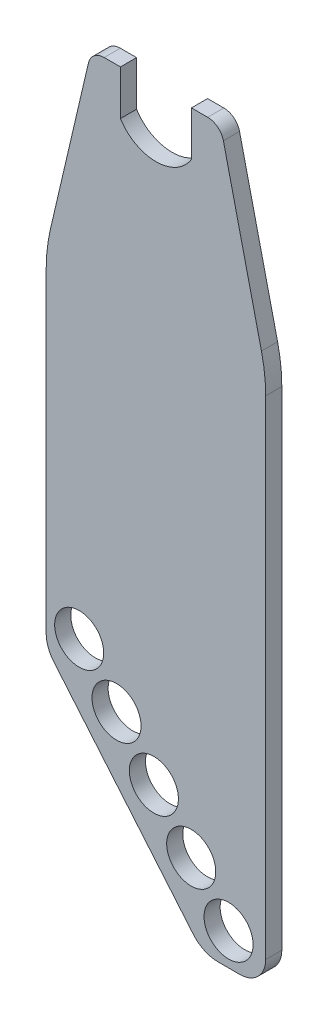
from build123d import *

# Parameters (mm, degrees)
SKETCH1_W           = 68
SKETCH1_H           = 225
BOSS_EXTRUDE1_DEPTH = 5
SKETCH3_R           = 7.6
CUT_EXTRUDE1_DEPTH  = 8
FILLET1_R           = 8
CUT_EXTRUDE2_DEPTH  = 118.631840928
FILLET2_R           = 10
CUT_EXTRUDE3_DEPTH  = 8
FILLET3_R           = 10
CUT_EXTRUDE4_DEPTH  = 118.631840928
FILLET4_R           = 5
FILLET5_R           = 50


with BuildPart() as part:
    # Sketch1 → Boss-Extrude1 (new body)
    with BuildSketch(Plane.XY):
        Rectangle(SKETCH1_W, SKETCH1_H)
    extrude(amount=BOSS_EXTRUDE1_DEPTH)

    # Sketch3 → Cut-Extrude1 (cut)
    with BuildSketch(Plane.XY.offset(5)):
        with Locations((22.5, -102.5)):
            Circle(SKETCH3_R)
        with Locations((10.929823026, -88.711200024)):
            Circle(SKETCH3_R)
        with Locations((-0.640353949, -74.922400048)):
            Circle(SKETCH3_R)
        with Locations((-12.210530923, -61.133600072)):
            Circle(SKETCH3_R)
        with Locations((-23.780707897, -47.344800095)):
            Circle(SKETCH3_R)
    extrude(amount=-CUT_EXTRUDE1_DEPTH, mode=Mode.SUBTRACT)

    # Fillet1
    fillet1_edges = [part.edges().sort_by_distance(p)[0] for p in [
        (34, -112.5, 2.5),
    ]]
    fillet(fillet1_edges, radius=FILLET1_R)

    # Sketch5 → Cut-Extrude2 (cut, through all)
    with BuildSketch(Plane.XY.offset(5)):
        Polygon((14.573405195, -112.5), (-34, -54.612469854), (-34, -112.5), align=None)
    extrude(amount=-CUT_EXTRUDE2_DEPTH, mode=Mode.SUBTRACT)

    # Fillet2
    fillet2_edges = [part.edges().sort_by_distance(p)[0] for p in [
        (14.573405195, -112.5, 2.5),
    ]]
    fillet(fillet2_edges, radius=FILLET2_R)

    # Sketch6 → Cut-Extrude3 (cut)
    with BuildSketch(Plane.XY.offset(5)):
        with BuildLine():
            Line((-11, 112.5), (-11, 98.643593539))
            ThreePointArc((-11, 98.643593539), (0, 92.57179677), (11, 98.643593539))
            Line((11, 98.643593539), (11, 112.5))
            ThreePointArc((11, 112.5), (0, 118.57179677), (-11, 112.5))
        make_face()
    extrude(amount=-CUT_EXTRUDE3_DEPTH, mode=Mode.SUBTRACT)

    # Fillet3
    fillet3_edges = [part.edges().sort_by_distance(p)[0] for p in [
        (-34, -54.612469854, 2.5),
    ]]
    fillet(fillet3_edges, radius=FILLET3_R)

    # Sketch7 → Cut-Extrude4 (cut, through all)
    with BuildSketch(Plane.XY.offset(5)):
        Polygon((-20, 112.5), (-34, 52.5), (-34, 112.5), align=None)
        Polygon((34, 112.5), (20, 112.5), (34, 52.5), align=None)
    extrude(amount=-CUT_EXTRUDE4_DEPTH, mode=Mode.SUBTRACT)

    # Fillet4
    fillet4_edges = [part.edges().sort_by_distance(p)[0] for p in [
        (20, 112.5, 2.5),
        (-20, 112.5, 2.5),
    ]]
    fillet(fillet4_edges, radius=FILLET4_R)

    # Fillet5
    fillet5_edges = [part.edges().sort_by_distance(p)[0] for p in [
        (34, 52.5, 2.5),
        (-34, 52.5, 2.5),
    ]]
    fillet(fillet5_edges, radius=FILLET5_R)


solid = part.part
